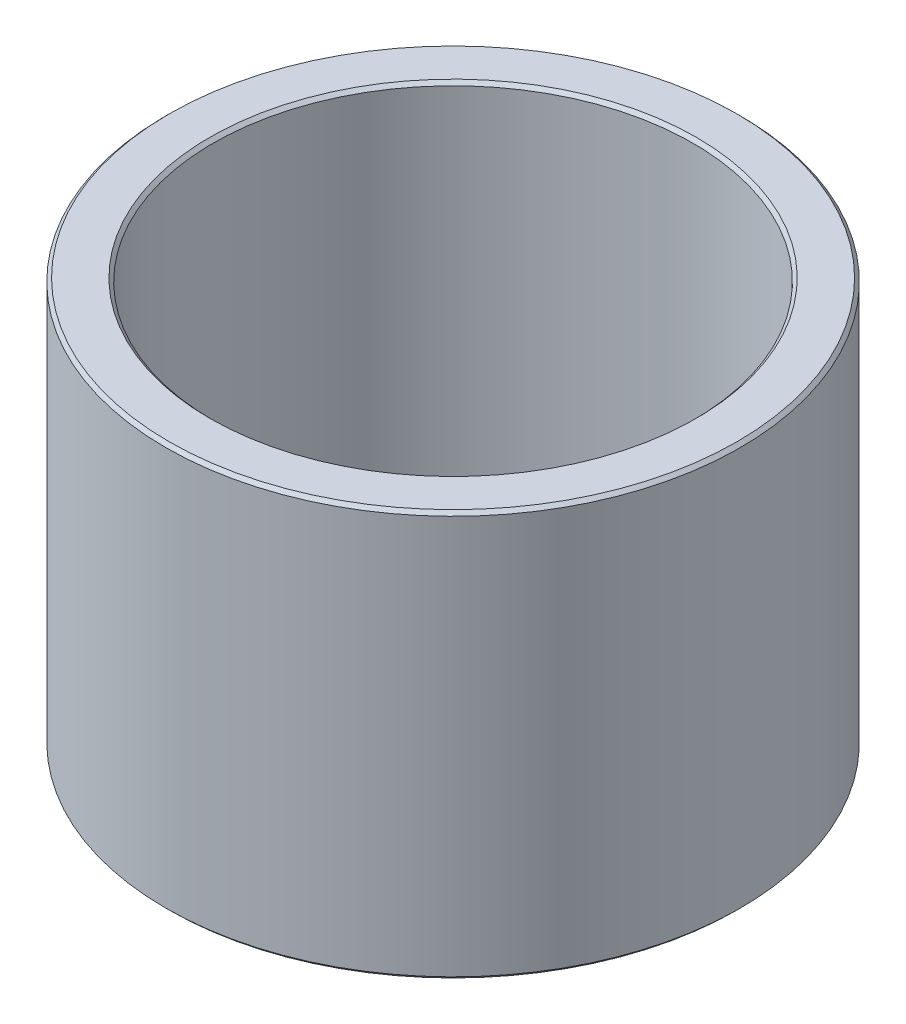
from build123d import *

# Parameters (mm, degrees)
SKETCH1_R           = 42.5
SKETCH1_R_2         = 35.5
BOSS_EXTRUDE1_DEPTH = 60
CHAMFER1_SIZE       = 0.5


with BuildPart() as part:
    # Sketch1 → Boss-Extrude1 (new body)
    with BuildSketch(Plane(origin=(0, 0, 0), x_dir=(1, 0, 0), z_dir=(0, 1, 0))):
        with Locations(Location((0, 0, 0), (0, 0, 270))):
            Circle(SKETCH1_R)
        with Locations(Location((0, 0, 0), (0, 0, 270))):
            Circle(SKETCH1_R_2, mode=Mode.SUBTRACT)
    extrude(amount=BOSS_EXTRUDE1_DEPTH)

    # Chamfer1
    chamfer1_edges = [part.edges().sort_by_distance(p)[0] for p in [
        (0, 0, -42.5),
        (0, 60, -42.5),
        (0, 0, -35.5),
        (0, 60, -35.5),
    ]]
    chamfer(chamfer1_edges, length=CHAMFER1_SIZE)


solid = part.part
